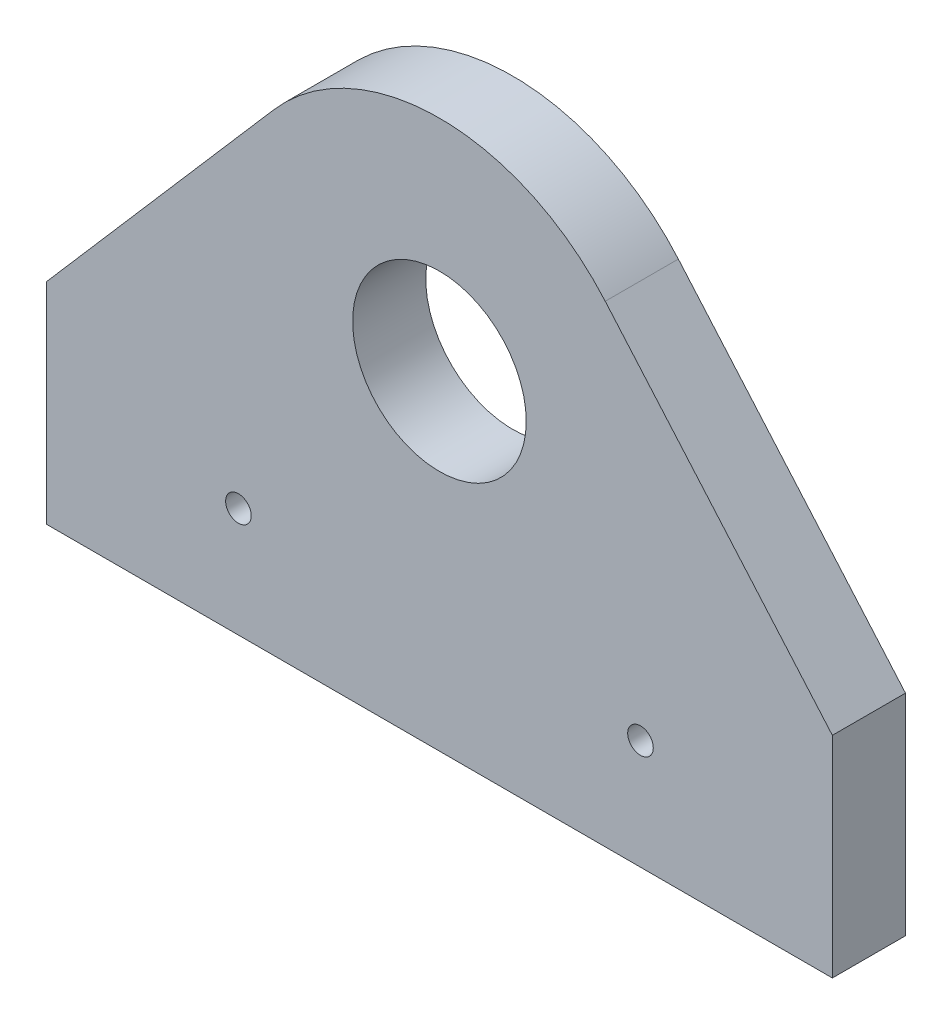
SolidWorks part; units mm, degrees
material "Q235"
ref_plane "Front Plane" through (0, 0, 0) normal (0, 0, 1) x (1, 0, 0)
ref_plane "Top Plane" through (0, 0, 0) normal (0, 1, 0) x (1, 0, 0)
ref_plane "Right Plane" through (0, 0, 0) normal (1, 0, 0) x (0, 0, -1)
sketch "Sketch1" plane through (0, 0, 0) normal (0, 0, 1) x (1, 0, 0)
  line L0 (0, 0) -> (0, -180) construction
  line L1 (-215, -180) -> (215, -180)
  line L4 (-90.723, 78.5452) -> (-215, -65)
  line L5 (90.723, 78.5452) -> (215, -65)
  line L6 (-215, -65) -> (-215, -180)
  line L7 (215, -65) -> (215, -180)
  line L8 (-215, -65) -> (215, -65) construction
  arc A0 (90.723, 78.5452) -> (-90.723, 78.5452) centre (0, 0) ccw
  dimension "D1" = 240
  dimension "D2" = 430
  dimension "D3" = 115
  dimension "D4" = 180
extrude "Boss-Extrude1" add sketch "Sketch1" along normal blind 40
sketch "Sketch2" plane through (0, 0, 40) normal (0, 0, 1) x (1, 0, 0)
  circle A0 centre (0, 0) radius 47.5
  dimension "D1" = 95
extrude "Cut-Extrude1" cut sketch "Sketch2" against normal through all
hole_wizard "M16 Tapped Hole1" positions "Sketch3" profile "Sketch4" tap size "M16" standard "GB" end condition through all
sketch "Sketch3" plane through (0, 0, 40) normal (0, 0, 1) x (1, 0, 0)
  line L0 (-110, -120) -> (110, -120) construction
  line L3 (0, -120) -> (0, -180) construction
  line L4 (-215, -180) -> (215, -180) construction
  point P0 (-110, -120)
  point P2 (110, -120)
  dimension "D1" = 220
  dimension "D2" = 60
sketch "Sketch4" plane through (-110, -120, 40) normal (1, 0, 0) x (0, -1, 0)
  line L0 (0, 0) -> (0, 40)
  line L1 (0, 40) -> (7, 40)
  line L2 (7, 40) -> (7, 0)
  line L5 (7, 0) -> (0, 0)
  line L11 (0, -6.35) -> (0, 107.95) construction
  dimension "通孔螺纹孔钻头直径" = 14
  dimension "通孔螺纹孔钻头深度" = 40
cosmetic thread "Hole thread 1" parameters "D2"=16
cosmetic thread "Hole thread 2" parameters "D2"=16
